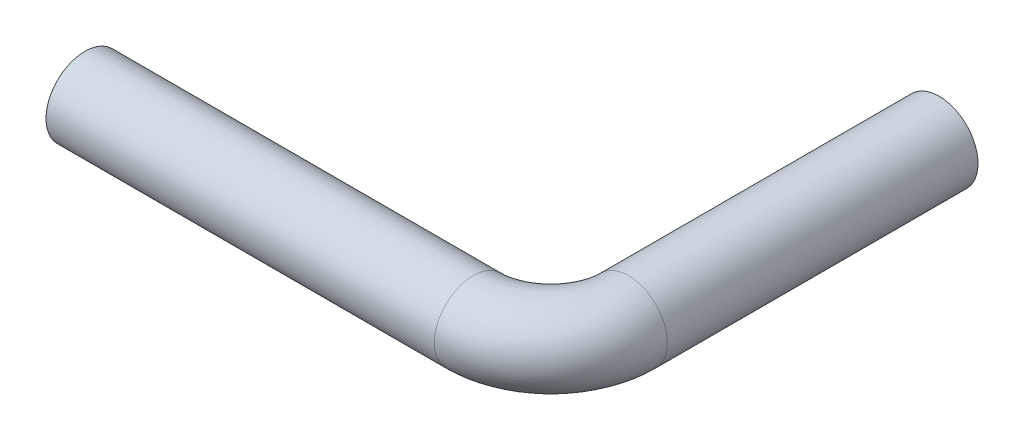
SolidWorks part; units mm, degrees
material "Plain Carbon Steel"
ref_plane "Front Plane" through (0, 0, 0) normal (0, 0, 1) x (1, 0, 0)
ref_plane "Top Plane" through (0, 0, 0) normal (0, 1, 0) x (1, 0, 0)
ref_plane "Right Plane" through (0, 0, 0) normal (1, 0, 0) x (0, 0, -1)
sketch "Sketch1" plane through (0, 0, 0) normal (0, 0, 1) x (1, 0, 0)
  circle A0 centre (0, 0) radius 2.5
  circle A1 centre (0, 0) radius 2
sketch "Sketch2" plane through (0, 0, 0) normal (0, 1, 0) x (1, 0, 0)
  line L0 (0, 0) -> (0, -20)
  line L1 (-5, -25) -> (-30, -25)
  arc A0 (0, -20) -> (-5, -25) centre (-5, -20) cw
  dimension "D1" = 5
sweep "Sweep1" add profiles "Sketch1" path "Sketch2"
